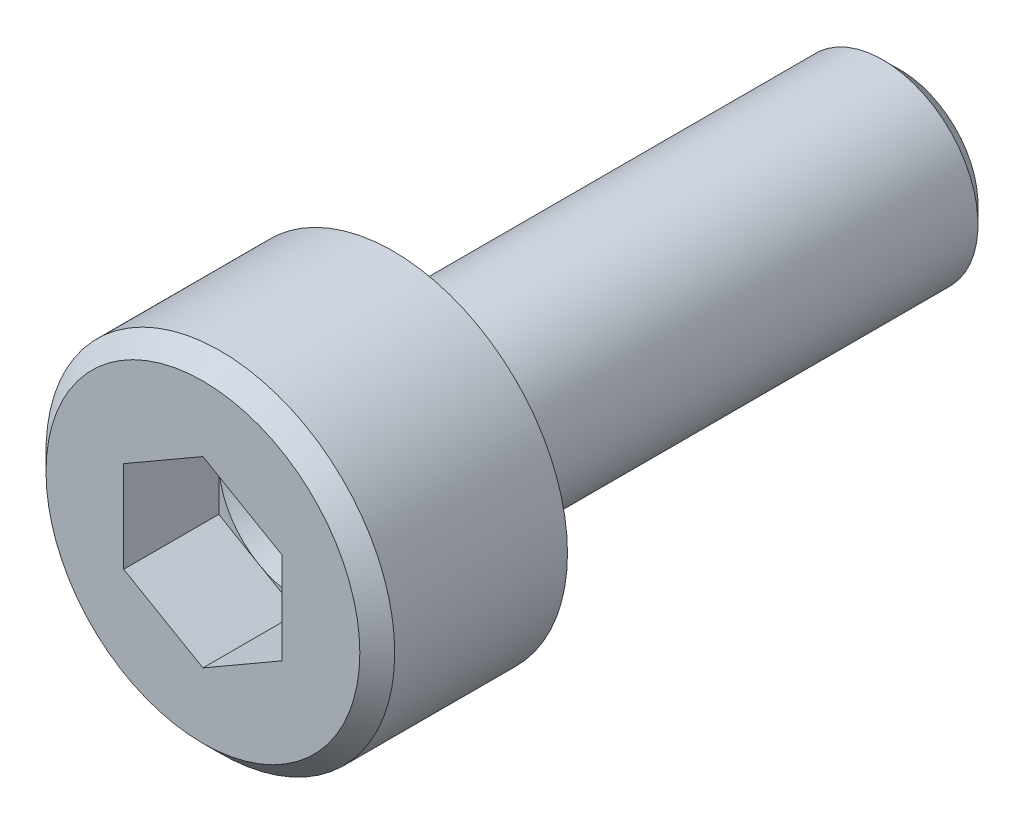
from build123d import *

# Parameters (mm, degrees)
SKETCH_1_W          = 2.75
SKETCH_1_H          = 3
SKETCH_2_R          = 1.5
EXTRUDE_1_DEPTH     = 8
CUT_EXTRUDE_1_DEPTH = 1.5
CHAMFER_1_SIZE      = 0.275


with BuildPart() as part:
    # 草图1 → 旋转1 (revolve)
    with BuildSketch(Plane(origin=(0, 0, 0), x_dir=(1, 0, 0), z_dir=(0, 1, 0))):
        with Locations((1.375, -1.5)):
            Rectangle(SKETCH_1_W, SKETCH_1_H)
    revolve(axis=Axis((0, 0, 0), (0, 0, 1)))

    # 草图2 → 凸台-拉伸1 (add)
    with BuildSketch(Plane(origin=(0, 0, 0), x_dir=(-1, 0, 0), z_dir=(0, 0, -1))):
        Circle(SKETCH_2_R)
    extrude(amount=EXTRUDE_1_DEPTH)

    # 草图3 → 切除-拉伸1 (cut)
    with BuildSketch(Plane.XY.offset(3)):
        Polygon((1.25, -0.721687836), (1.25, 0.721687836), (0, 1.443375673), (-1.25, 0.721687836), (-1.25, -0.721687836), (0, -1.443375673), align=None)
    extrude(amount=-CUT_EXTRUDE_1_DEPTH, mode=Mode.SUBTRACT)

    # 草图4 → 切除-旋转1 (revolve, cut)
    with BuildSketch(Plane.XZ):
        Polygon((1.25, 1.5), (0, 1.5), (0, 0.778312164), align=None)
    revolve(axis=Axis((0, 0, 1.5), (0, 0, -1)), mode=Mode.SUBTRACT)

    # 倒角1
    chamfer_1_edges = [part.edges().sort_by_distance(p)[0] for p in [
        (-2.75, 0, 3),
        (1.5, 0, -8),
    ]]
    chamfer(chamfer_1_edges, length=CHAMFER_1_SIZE)


solid = part.part
